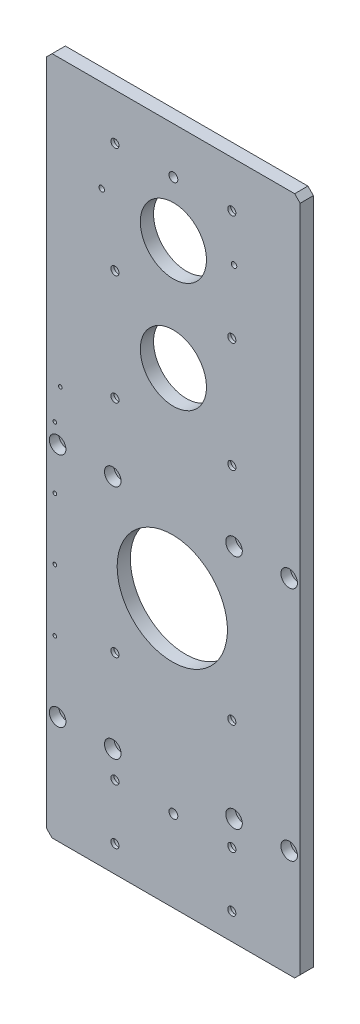
SolidWorks part; units mm, degrees
material "6061-T6"
ref_plane "前视基准面" through (0, 0, 0) normal (0, 0, 1) x (1, 0, 0)
ref_plane "上视基准面" through (0, 0, 0) normal (0, 1, 0) x (1, 0, 0)
ref_plane "右视基准面" through (0, 0, 0) normal (1, 0, 0) x (0, 0, -1)
sketch "草图1" plane through (0, 0, 0) normal (0, 0, 1) x (1, 0, 0)
  line L1 (210.0261, 629.8574) -> (-19.9739, 629.8574)
  line L2 (210.0261, 629.8574) -> (210.0261, 13.8574)
  line L3 (210.0261, 13.8574) -> (-19.9739, 13.8574)
  line L4 (-19.9739, 629.8574) -> (-19.9739, 13.8574)
  dimension "D1" = 230
  dimension "D2" = 616
extrude "凸台-拉伸1" add sketch "草图1" along normal blind 12
chamfer "倒角1" distance 5 angle 45 4 edges at (-19.9739, 13.8574, 6) (210.0261, 13.8574, 6) (-19.9739, 629.8574, 6) (210.0261, 629.8574, 6)
hole_wizard "M8 六角凹头螺钉的柱形沉头孔1" positions "草图2" profile "草图3" counterbore size "M8" standard "ISO"
sketch "草图2" plane through (0, 0, 0) normal (0, 0, -1) x (-1, 0, 0)
  point P0 (-148.0261, 587.8574)
  point P2 (-42.0261, 587.8574)
  point P4 (-148.0261, 487.8574)
  point P6 (-42.0261, 487.8574)
  point P8 (-148.0261, 387.8574)
  point P10 (-42.0261, 387.8574)
  point P12 (-148.0261, 187.8574)
  point P14 (-42.0261, 187.8574)
  point P16 (-148.0261, 87.8574)
  point P18 (-42.0261, 87.8574)
  point P20 (-148.0261, 37.8574)
  point P22 (-42.0261, 37.8574)
sketch "草图3" plane through (148.0261, 587.8574, 0) normal (1, 0, 0) x (0, 1, 0)
  line L0 (0, 0) -> (0, 14.2039)
  line L1 (0, 14.2039) -> (4.5, 11.5)
  line L2 (4.5, 11.5) -> (4.5, 8.6)
  line L3 (4.5, 8.6) -> (7.5, 8.6)
  line L4 (7.5, 8.6) -> (7.5, 0)
  line L5 (7.5, 0) -> (0, 0)
  line L10 (0, 14.2039) -> (-4.5, 11.5) construction
  line L11 (0, -6.35) -> (0, 107.95) construction
  dimension "孔直径" = 9
  dimension "孔深度" = 11.5
  dimension "柱形沉头孔直径" = 15
  dimension "柱形沉头孔深度" = 8.6
  dimension "导头角度" = 118
hole_wizard "M8 六角凹头螺钉的柱形沉头孔2" positions "草图4" profile "草图5" counterbore size "M8" standard "ISO"
sketch "草图4" plane through (0, 0, 12) normal (0, 0, 1) x (1, 0, 0)
  point P0 (-9.9739, 325.3574)
  point P2 (40.0261, 325.3574)
  point P4 (150.0261, 325.3574)
  point P6 (200.0261, 325.3574)
  point P8 (-9.9739, 111.3574)
  point P10 (40.0261, 111.3574)
  point P12 (150.0261, 111.3574)
  point P14 (200.0261, 111.3574)
sketch "草图5" plane through (-9.9739, 325.3574, 12) normal (1, 0, 0) x (0, -1, 0)
  line L0 (0, 0) -> (0, 24.9539)
  line L1 (0, 24.9539) -> (4.5, 22.25)
  line L2 (4.5, 22.25) -> (4.5, 8.6)
  line L3 (4.5, 8.6) -> (7.5, 8.6)
  line L4 (7.5, 8.6) -> (7.5, 0)
  line L5 (7.5, 0) -> (0, 0)
  line L10 (0, 24.9539) -> (-4.5, 22.25) construction
  line L11 (0, -6.35) -> (0, 107.95) construction
  dimension "孔直径" = 9
  dimension "孔深度" = 22.25
  dimension "柱形沉头孔直径" = 15
  dimension "柱形沉头孔深度" = 8.6
  dimension "导头角度" = 118
hole_wizard "大小mm 暗销孔1" positions "草图6" profile "草图7" hole size "Ø8.0" standard "ISO"
sketch "草图6" plane through (0, 0, 12) normal (0, 0, 1) x (1, 0, 0)
  point P0 (95.0261, 587.8574)
  point P2 (95.0261, 87.8574)
sketch "草图7" plane through (95.0261, 587.8574, 12) normal (1, 0, 0) x (0, -1, 0)
  line L0 (0, 0) -> (0, 24.6534)
  line L1 (0, 24.6534) -> (4, 22.25)
  line L2 (4, 22.25) -> (4, 0)
  line L5 (4, 0) -> (0, 0)
  line L10 (0, 24.6534) -> (-4, 22.25) construction
  line L11 (0, -6.35) -> (0, 107.95) construction
  dimension "孔直径" = 8
  dimension "孔深度" = 22.25
  dimension "导头角度" = 118
hole_wizard "M4 螺纹孔1" positions "草图8" profile "草图9" tap size "M4" standard "ISO" end condition through all
sketch "草图8" plane through (0, 0, 12) normal (0, 0, 1) x (1, 0, 0)
  point P0 (-12.4739, 341.8574)
  point P2 (-12.4739, 285.8574)
  point P4 (-12.4739, 229.8574)
  point P6 (-12.4739, 173.8574)
sketch "草图9" plane through (-12.4739, 341.8574, 12) normal (1, 0, 0) x (0, -1, 0)
  line L0 (0, 0) -> (0, 12)
  line L1 (0, 12) -> (1.65, 12)
  line L2 (1.65, 12) -> (1.65, 0)
  line L5 (1.65, 0) -> (0, 0)
  line L11 (0, -6.35) -> (0, 107.95) construction
  dimension "通孔螺纹孔钻头直径" = 3.3
  dimension "通孔螺纹孔钻头深度" = 12
cosmetic thread "孔螺蚊线1" parameters "D2"=4
cosmetic thread "孔螺蚊线2" parameters "D2"=4
cosmetic thread "孔螺蚊线3" parameters "D2"=4
cosmetic thread "孔螺蚊线4" parameters "D2"=4
hole_wizard "M4 螺纹孔2" positions "草图10" profile "草图11" tap size "M4" standard "ISO" end condition through all
sketch "草图10" plane through (0, 0, 12) normal (0, 0, 1) x (1, 0, 0)
  point P0 (-7.4739, 371.8574)
sketch "草图11" plane through (-7.4739, 371.8574, 12) normal (1, 0, 0) x (0, -1, 0)
  line L0 (0, 0) -> (0, 12)
  line L1 (0, 12) -> (1.65, 12)
  line L2 (1.65, 12) -> (1.65, 0)
  line L5 (1.65, 0) -> (0, 0)
  line L11 (0, -6.35) -> (0, 107.95) construction
  dimension "通孔螺纹孔钻头直径" = 3.3
  dimension "通孔螺纹孔钻头深度" = 12
cosmetic thread "孔螺蚊线5" parameters "D2"=4
sketch "草图12" plane through (0, 0, 0) normal (0, 0, -1) x (-1, 0, 0)
  line L0 (-148.0261, 587.8574) -> (-42.0261, 487.8574) construction
  line L1 (-148.0261, 387.8574) -> (-42.0261, 487.8574) construction
  line L2 (-148.0261, 187.8574) -> (-40.0261, 325.3574) construction
  circle A0 centre (-95.0261, 537.8574) radius 30
  circle A1 centre (-95.0261, 437.8574) radius 30
  circle A2 centre (-94.0261, 256.6074) radius 50
  dimension "D1" = 60
  dimension "D2" = 100
extrude "切除-拉伸1" cut sketch "草图12" against normal through all
hole_wizard "M6 螺纹孔1" positions "草图15" profile "草图16" tap size "M6" standard "ISO"
sketch "草图15" plane through (0, 0, 0) normal (0, 0, -1) x (-1, 0, 0)
  line L0 (-150.0261, 546.3574) -> (-30.0261, 546.3574) construction
  line L2 (19.9739, 624.8574) -> (19.9739, 18.8574) construction
  line L3 (-205.0261, 629.8574) -> (14.9739, 629.8574) construction
  point P0 (-150.0261, 546.3574)
  point P2 (-30.0261, 546.3574)
  dimension "D1" = 120
  dimension "D2" = 50
  dimension "D3" = 83.5
sketch "草图16" plane through (150.0261, 546.3574, 0) normal (1, 0, 0) x (0, 1, 0)
  line L0 (0, 0) -> (0, 18.5022)
  line L1 (0, 18.5022) -> (2.5, 17)
  line L2 (2.5, 17) -> (2.5, 0)
  line L5 (2.5, 0) -> (0, 0)
  line L10 (0, 18.5022) -> (-2.5, 17) construction
  line L11 (0, -6.35) -> (0, 107.95) construction
  dimension "螺纹孔钻头直径" = 5
  dimension "螺纹孔钻头深度" = 17
  dimension "导头角度" = 118
cosmetic thread "孔螺蚊线8"
cosmetic thread "孔螺蚊线9"
